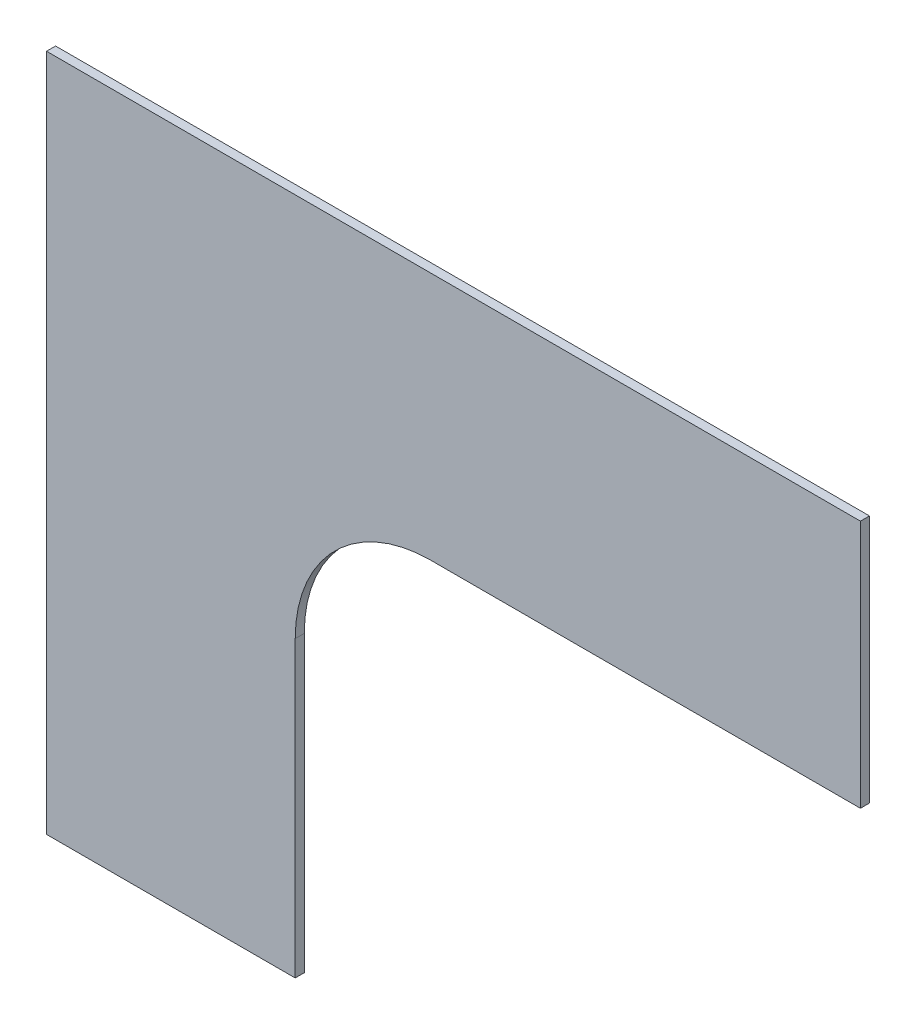
from build123d import *

# Parameters (mm, degrees)
BOSS_EXTRUDE1_DEPTH = 20


with BuildPart() as part:
    # Sketch1 → Boss-Extrude1 (new body)
    with BuildSketch(Plane.XY):
        with BuildLine():
            Line((0, 0), (0, 1500))
            Line((0, 1500), (1800, 1500))
            Line((1800, 1500), (1800, 950))
            Line((1800, 950), (850, 950))
            ThreePointArc((850, 950), (637.867965644, 862.132034356), (550, 650))
            Line((550, 650), (550, 0))
            Line((550, 0), (0, 0))
        make_face()
    extrude(amount=BOSS_EXTRUDE1_DEPTH)


solid = part.part
